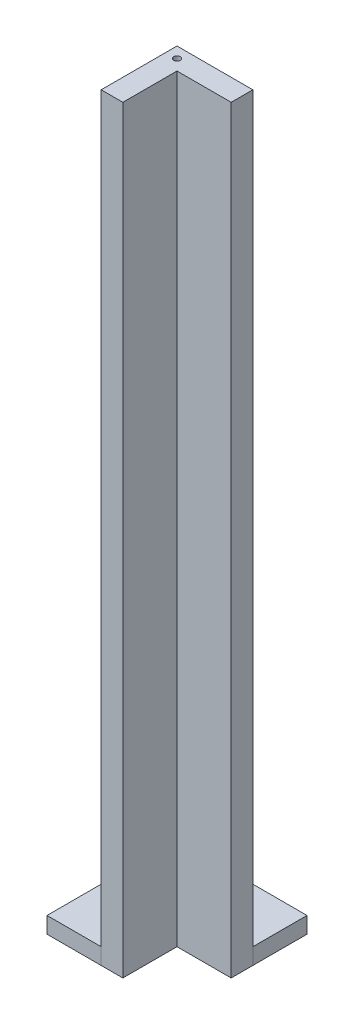
from build123d import *

# Parameters (mm, degrees)
SKETCH2_R                = 8
BOSS_EXTRUDE1_DEPTH      = 15
BOSS_EXTRUDE2_DEPTH      = 685
BOSS_EXTRUDE2_DEPTH_BACK = 15
SKETCH4_R                = 3
CUT_EXTRUDE1_DEPTH       = 20


with BuildPart() as part:
    # Sketch2 → Boss-Extrude1 (new body)
    with BuildSketch(Plane(origin=(0, 0, 0), x_dir=(1, 0, 0), z_dir=(0, 1, 0))):
        Polygon((-60, -60), (-10, -60), (-10, 10), (60, 10), (60, 60), (-60, 60), align=None)
        with Locations(Location((-35, -10, 0), (0, 0, 270))):
            Circle(SKETCH2_R, mode=Mode.SUBTRACT)
        with Locations(Location((10, 35, 0), (0, 0, 270))):
            Circle(SKETCH2_R, mode=Mode.SUBTRACT)
    extrude(amount=BOSS_EXTRUDE1_DEPTH)


with BuildPart() as body_2:
    # Sketch3 → Boss-Extrude2 (new, two sides: drawn at the far end of the back side and taken through both)
    with BuildSketch(Plane(origin=(0, 15, 0), x_dir=(1, 0, 0), z_dir=(0, 1, 0)).offset(-BOSS_EXTRUDE2_DEPTH_BACK)):
        Polygon((-10, -60), (-10, 10), (60, 10), (60, -10), (10, -10), (10, -60), align=None)
    extrude(amount=BOSS_EXTRUDE2_DEPTH + BOSS_EXTRUDE2_DEPTH_BACK)

    # Sketch4 → Cut-Extrude1 (cut)
    with BuildSketch(Plane(origin=(0, 700, 0), x_dir=(1, 0, 0), z_dir=(0, 1, 0))):
        with Locations(Location((0, 0, 0), (0, 0, 270))):
            Circle(SKETCH4_R)
    extrude(amount=-CUT_EXTRUDE1_DEPTH, mode=Mode.SUBTRACT)


solid = Compound([part.part, body_2.part])
